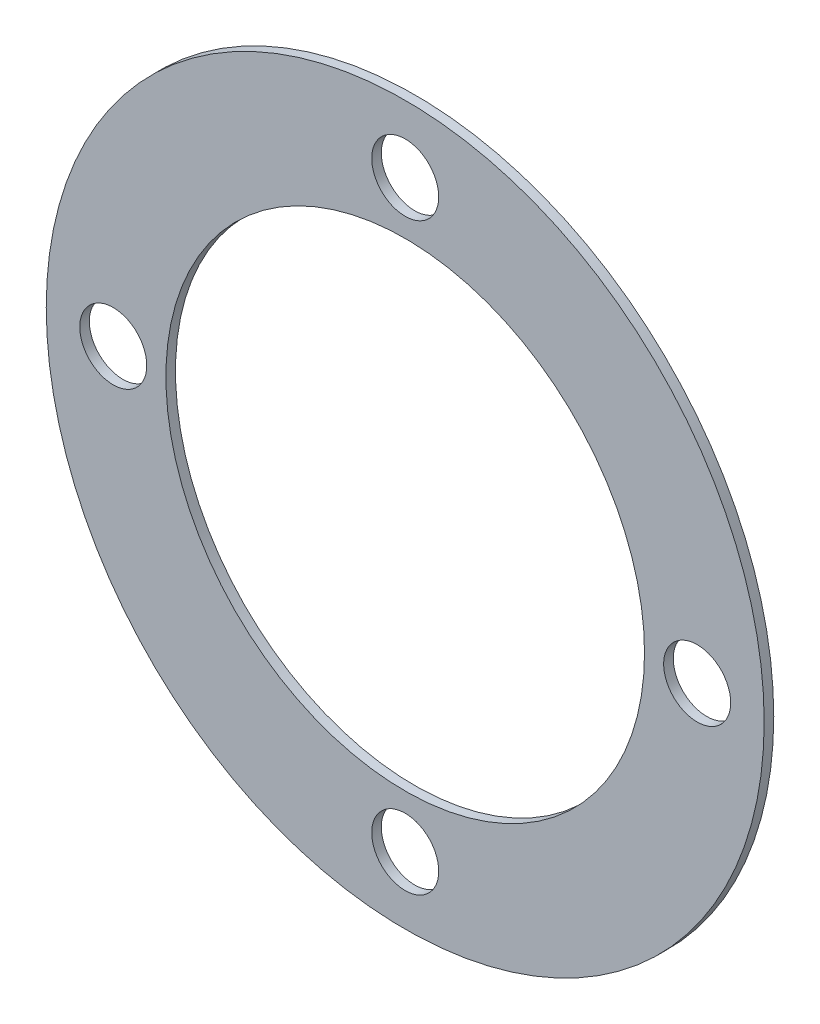
SolidWorks part; units mm, degrees
ref_plane "Front Plane" through (0, 0, 0) normal (0, 0, 1) x (1, 0, 0)
ref_plane "Top Plane" through (0, 0, 0) normal (0, 1, 0) x (1, 0, 0)
ref_plane "Right Plane" through (0, 0, 0) normal (1, 0, 0) x (0, 0, -1)
other "Configuration Table"
sketch "Sketch1" plane through (0, 0, 0) normal (0, 0, 1) x (1, 0, 0)
  line L0 (0, 0) -> (0, 43.6093) construction
  circle A0 centre (0, 0) radius 25
  circle A1 centre (0, 0) radius 37.5
  circle A2 centre (0, 30.5) radius 3.5
  circle A3 centre (30.5, 0) radius 3.5
  circle A4 centre (0, -30.5) radius 3.5
  circle A5 centre (-30.5, 0) radius 3.5
  point P16 (0, 0)
  dimension "D1" = 75
  dimension "D2" = 50
  dimension "D3" = 7
  dimension "D4" = 30.5
  dimension "D5" = 4
extrude "Boss-Extrude1" add sketch "Sketch1" along normal blind 1
